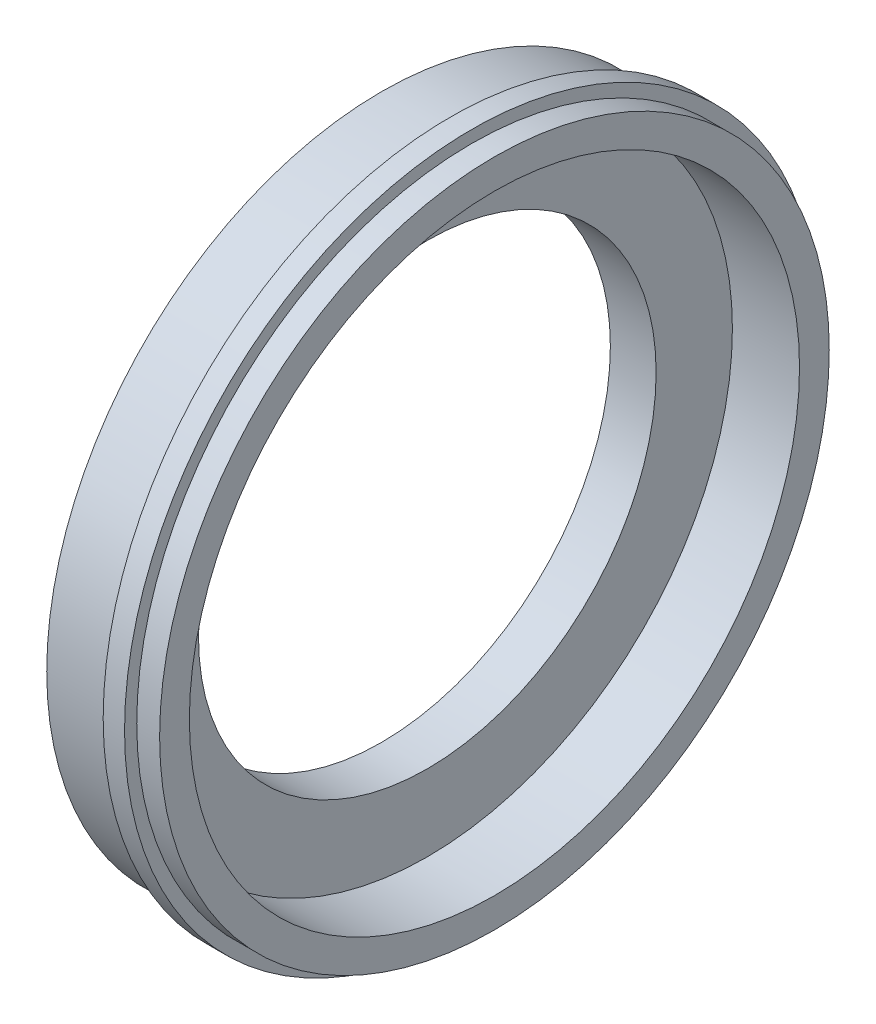
SolidWorks part; units mm, degrees
material "灰铸铁 HT150 "
ref_plane "Front Plane" through (0, 0, 0) normal (0, 0, 1) x (1, 0, 0)
ref_plane "Top Plane" through (0, 0, 0) normal (0, 1, 0) x (1, 0, 0)
ref_plane "Right Plane" through (0, 0, 0) normal (1, 0, 0) x (0, 0, -1)
sketch "Sketch1" plane through (0, 0, 0) normal (0, 1, 0) x (1, 0, 0)
  line L0 (0, 0) -> (212.6126, 0) construction
  line L1 (0, 150) -> (0, 163)
  line L2 (0, 219.5) -> (45, 219.5)
  line L3 (45, 219.5) -> (45, 227.5)
  line L4 (45, 227.5) -> (59, 227.5)
  line L5 (59, 227.5) -> (59, 219.5)
  line L6 (59, 219.5) -> (74, 219.5)
  line L7 (74, 219.5) -> (74, 200)
  line L8 (74, 200) -> (30, 200)
  line L9 (30, 200) -> (30, 150)
  line L10 (30, 150) -> (0, 150)
  line L15 (0, 203) -> (0, 219.5)
  line L16 (0, 203) -> (14, 203)
  line L17 (0, 189) -> (14, 189)
  line L18 (14, 203) -> (14, 189)
  line L19 (0, 177) -> (0, 189)
  line L20 (0, 177) -> (14, 177)
  line L21 (0, 163) -> (14, 163)
  line L22 (14, 177) -> (14, 163)
  dimension "D1" = 150
  dimension "D2" = 163
  dimension "D3" = 177
  dimension "D4" = 189
  dimension "D5" = 203
  dimension "D6" = 219.5
  dimension "D7" = 14
  dimension "D8" = 227.5
  dimension "D9" = 14
  dimension "D10" = 29
  dimension "D11" = 74
  dimension "D12" = 200
  dimension "D13" = 30
revolve "Revolve1" add sketch "Sketch1" angle 360 about L0
